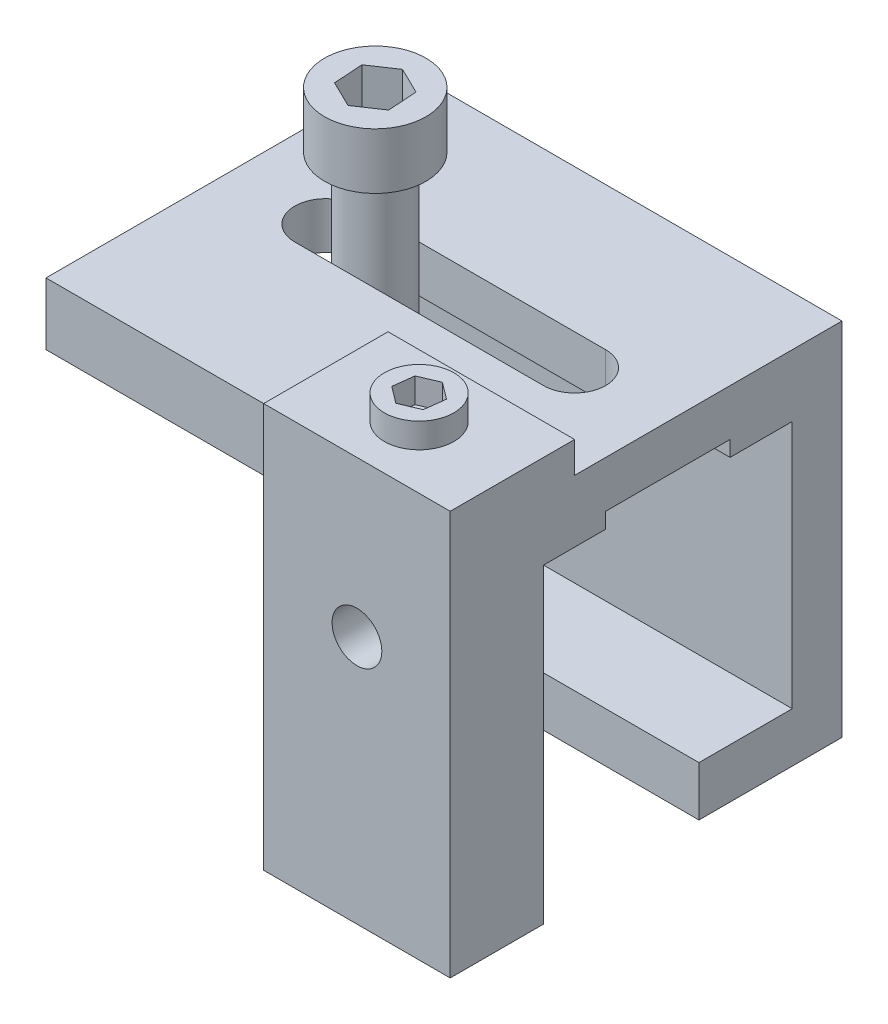
from build123d import *

# Parameters (mm, degrees)
SKETCH1_W                = 70
SKETCH1_H                = 50
BOSS_EXTRUDE1_DEPTH      = 10
SKETCH2_W                = 30
SKETCH2_H                = 10
BOSS_EXTRUDE2_DEPTH      = 50
SKETCH3_W                = 30
SKETCH3_H                = 15
BOSS_EXTRUDE3_DEPTH      = 5
SKETCH4_W                = 30
SKETCH4_H                = 65
BOSS_EXTRUDE4_DEPTH      = 5
CUT_EXTRUDE1_DEPTH       = 10
CUT_EXTRUDE2_REACH       = 104.103
SKETCH6_W                = 20
SKETCH6_H                = 5
SKETCH7_R                = 5.585417207
BOSS_EXTRUDE5_DEPTH      = 4
CUT_EXTRUDE3_REACH       = 104.103
SKETCH8_R                = 4
BOSS_EXTRUDE6_DEPTH      = 4
BOSS_EXTRUDE6_DEPTH_BACK = 24
SKETCH9_R                = 5
SKETCH10_R               = 8.158822916
BOSS_EXTRUDE7_DEPTH      = 9
CUT_EXTRUDE4_DEPTH       = 7
BOSS_EXTRUDE8_DEPTH      = 70


with BuildPart() as part:
    # Sketch1 → Boss-Extrude1 (new body)
    with BuildSketch(Plane(origin=(0, 0, 0), x_dir=(1, 0, 0), z_dir=(0, 1, 0))):
        with Locations((35, -25)):
            Rectangle(SKETCH1_W, SKETCH1_H)
    extrude(amount=BOSS_EXTRUDE1_DEPTH)

    # Sketch2 → Boss-Extrude2 (add)
    with BuildSketch(Plane.XZ):
        with Locations((55, 45)):
            Rectangle(SKETCH2_W, SKETCH2_H)
    extrude(amount=BOSS_EXTRUDE2_DEPTH)

    # Sketch3 → Boss-Extrude3 (add)
    with BuildSketch(Plane(origin=(0, 10, 0), x_dir=(1, 0, 0), z_dir=(0, 1, 0))):
        with Locations((55, -42.5)):
            Rectangle(SKETCH3_W, SKETCH3_H)
    extrude(amount=BOSS_EXTRUDE3_DEPTH)

    # Sketch4 → Boss-Extrude4 (add)
    with BuildSketch(Plane.XY.offset(50)):
        with Locations((55, -17.5)):
            Rectangle(SKETCH4_W, SKETCH4_H)
    extrude(amount=BOSS_EXTRUDE4_DEPTH)

    # Sketch5 → Cut-Extrude1 (cut)
    with BuildSketch(Plane(origin=(0, 10, 0), x_dir=(1, 0, 0), z_dir=(0, 1, 0))):
        with BuildLine():
            Line((15, -15), (55, -15))
            ThreePointArc((55, -15), (60, -20), (55, -25))
            Line((55, -25), (15, -25))
            ThreePointArc((15, -25), (10, -20), (15, -15))
        make_face()
    extrude(amount=-CUT_EXTRUDE1_DEPTH, mode=Mode.SUBTRACT)

    # Sketch6 → Cut-Extrude2 (cut, up to next)
    with BuildSketch(Plane.ZY, mode=Mode.PRIVATE) as cut_extrude2_sk1:
        with Locations((20, 0)):
            Rectangle(SKETCH6_W, SKETCH6_H)
    cut_extrude2_tool1 = extrude(cut_extrude2_sk1.sketch, amount=-CUT_EXTRUDE2_REACH, mode=Mode.PRIVATE) & part.part
    add(cut_extrude2_tool1.solids().sort_by_distance((0, 0, 20))[0], mode=Mode.SUBTRACT)

    # Sketch7 → Boss-Extrude5 (add)
    with BuildSketch(Plane(origin=(0, 15, 0), x_dir=(1, 0, 0), z_dir=(0, 1, 0))):
        with Locations(Location((55, -45, 0), (0, 0, 270))):
            Circle(SKETCH7_R)
        Polygon((57.67966577, -47.022225035), (58.091131137, -43.690453887), (55.411465367, -41.668228852), (52.32033423, -42.977774965), (51.908868863, -46.309546113), (54.588534633, -48.331771148), align=None, mode=Mode.SUBTRACT)
    extrude(amount=BOSS_EXTRUDE5_DEPTH)

    # Sketch8 → Cut-Extrude3 (cut, up to next)
    with BuildSketch(Plane.XY.offset(55), mode=Mode.PRIVATE) as cut_extrude3_sk1:
        with Locations((55, -10)):
            Circle(SKETCH8_R)
    cut_extrude3_tool1 = extrude(cut_extrude3_sk1.sketch, amount=-CUT_EXTRUDE3_REACH, mode=Mode.PRIVATE) & part.part
    add(cut_extrude3_tool1.solids().sort_by_distance((55, -10, 55))[0], mode=Mode.SUBTRACT)

    # Sketch12 → Boss-Extrude8 (add)
    with BuildSketch(Plane.ZY):
        Polygon((0, 10), (-8, 10), (-8, -48), (15, -48), (15, -40), (0, -40), align=None)
    extrude(amount=-BOSS_EXTRUDE8_DEPTH)


with BuildPart() as body_2:
    # Sketch9 → Boss-Extrude6 (new, two sides: drawn at the far end of the back side and taken through both)
    with BuildSketch(Plane.XZ.offset(-BOSS_EXTRUDE6_DEPTH_BACK)):
        with Locations(Location((22.947817681, 20, 0), (0, 0, 270))):
            Circle(SKETCH9_R)
    extrude(amount=BOSS_EXTRUDE6_DEPTH + BOSS_EXTRUDE6_DEPTH_BACK)

    # Sketch10 → Boss-Extrude7 (add)
    with BuildSketch(Plane(origin=(0, 24, 0), x_dir=(1, 0, 0), z_dir=(0, 1, 0))):
        with Locations(Location((22.947817681, -20, 0), (0, 0, 270))):
            Circle(SKETCH10_R)
    extrude(amount=BOSS_EXTRUDE7_DEPTH)

    # Sketch11 → Cut-Extrude4 (cut)
    with BuildSketch(Plane(origin=(0, 33, 0), x_dir=(1, 0, 0), z_dir=(0, 1, 0))):
        Polygon((27.183408911, -22.07074215), (26.858928603, -17.367241469), (22.623337372, -15.296499319), (18.71222645, -17.92925785), (19.036706759, -22.632758531), (23.272297989, -24.703500681), align=None)
    extrude(amount=-CUT_EXTRUDE4_DEPTH, mode=Mode.SUBTRACT)


solid = Compound([part.part, body_2.part])
